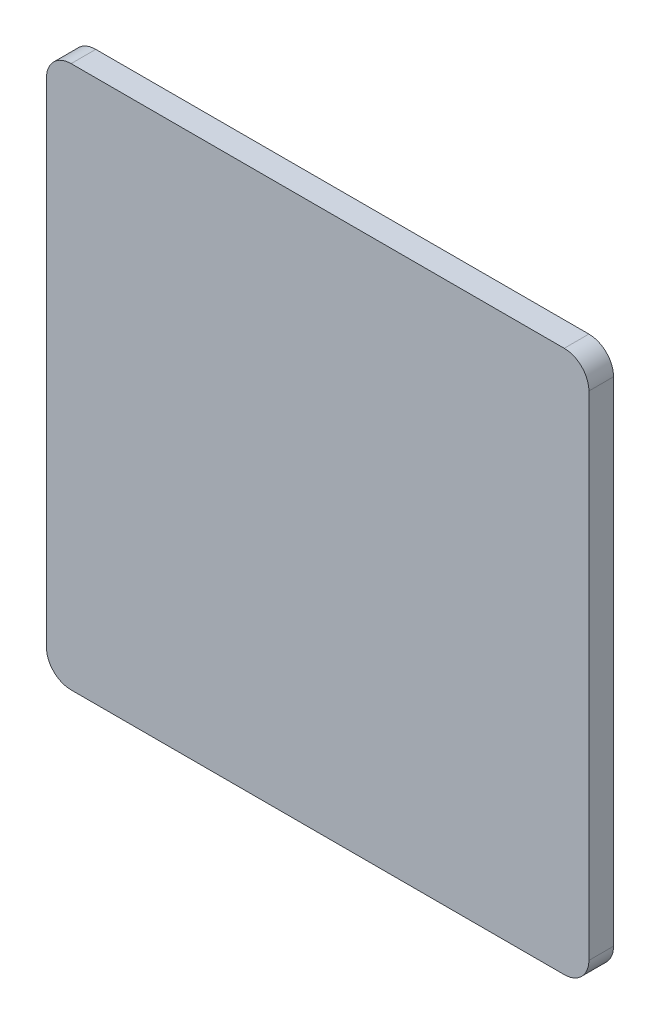
SolidWorks part; units mm, degrees
ref_plane "前视基准面" through (0, 0, 0) normal (0, 0, 1) x (1, 0, 0)
ref_plane "上视基准面" through (0, 0, 0) normal (0, 1, 0) x (1, 0, 0)
ref_plane "右视基准面" through (0, 0, 0) normal (1, 0, 0) x (0, 0, -1)
sketch "草图1" plane through (0, 0, 0) normal (0, 0, 1) x (1, 0, 0)
  line L1 (110, -110) -> (-110, -110)
  line L2 (110, -110) -> (110, 110)
  line L3 (110, 110) -> (-110, 110)
  line L4 (-110, -110) -> (-110, 110)
  line L5 (110, -110) -> (-110, 110) construction
  line L6 (110, 110) -> (-110, -110) construction
  point P0 (0, 0)
  dimension "D1" = 220
extrude "凸台-拉伸1" add sketch "草图1" along normal blind 10
fillet "圆角1" radius 10 4 edges at (110, -110, 5) (110, 110, 5) (-110, -110, 5) (-110, 110, 5)
